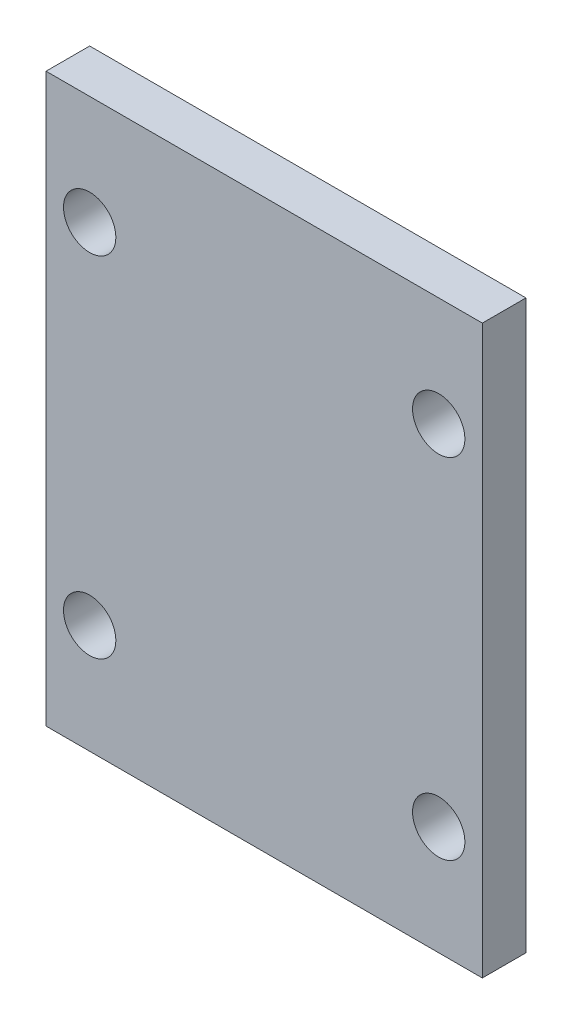
from build123d import *

# Parameters (mm, degrees)
SKETCH1_W           = 100
SKETCH1_H           = 130
BOSS_EXTRUDE1_DEPTH = 5
F_12_HOLE1_D        = 12


with BuildPart() as part:
    # Sketch1 → Boss-Extrude1 (new, symmetric)
    with BuildSketch(Plane.XY):
        Rectangle(SKETCH1_W, SKETCH1_H)
    extrude(amount=BOSS_EXTRUDE1_DEPTH, both=True)

    # Ø12 Hole1 (through all)
    with Locations(Plane.XY.offset(5)):
        with Locations((-40, 40), (40, 40), (40, -40), (-40, -40)):
            Hole(F_12_HOLE1_D / 2)


solid = part.part
